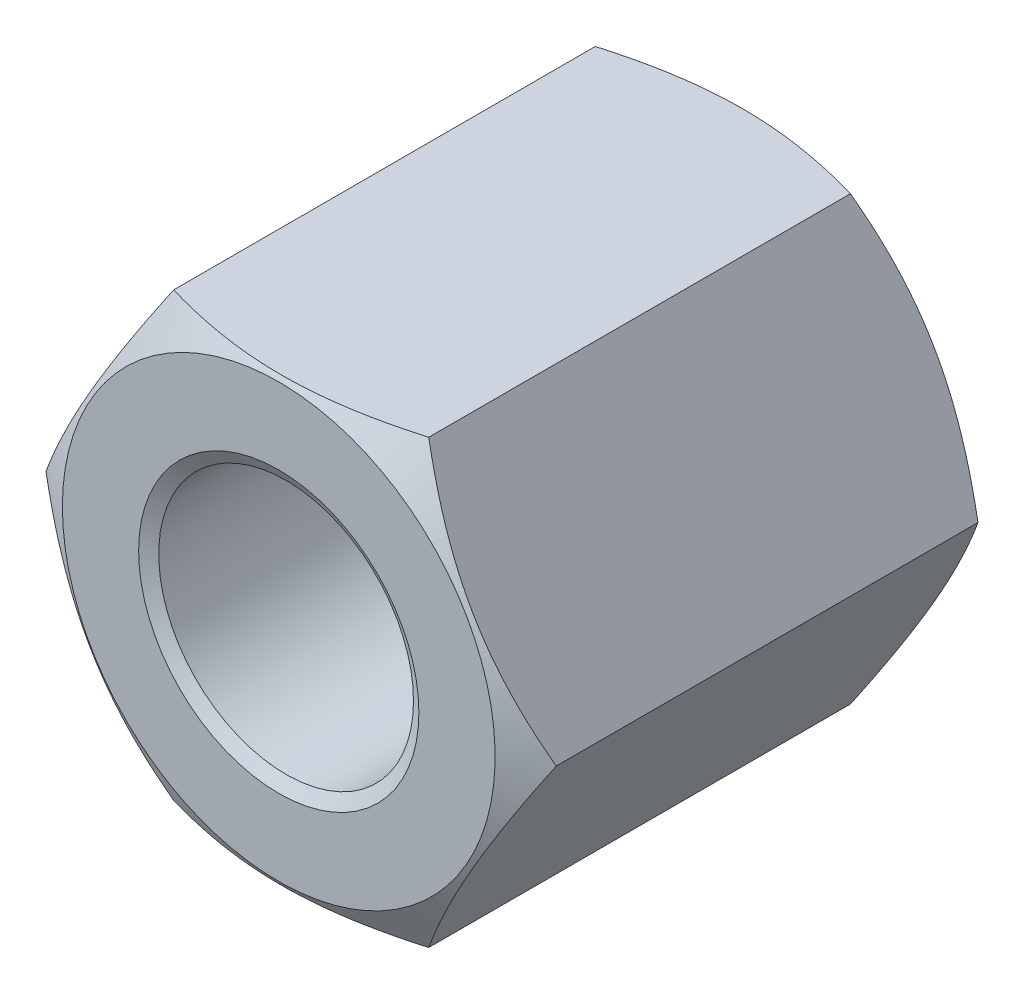
SolidWorks part; units mm, degrees
ref_plane "Front" through (0, 0, 0) normal (0, 0, 1) x (1, 0, 0)
ref_plane "Top" through (0, 0, 0) normal (0, 1, 0) x (1, 0, 0)
ref_plane "Right" through (0, 0, 0) normal (1, 0, 0) x (0, 0, -1)
other "Configuration Table"
sketch "Sketch1" plane through (0, 0, 0) normal (0, 0, 1) x (1, 0, 0)
  line L1 (10.3923, -18) -> (20.7846, 0)
  line L2 (20.7846, 0) -> (10.3923, 18)
  line L3 (10.3923, 18) -> (-10.3923, 18)
  line L4 (-10.3923, 18) -> (-20.7846, 0)
  line L5 (-20.7846, 0) -> (-10.3923, -18)
  line L6 (-10.3923, -18) -> (10.3923, -18)
  circle A0 centre (0, 0) radius 18 construction
  circle A1 centre (0, 0) radius 10.376
extrude "BaseNut" add sketch "Sketch1" against normal blind 38
cosmetic thread "ThreadCosmetic1" parameters "D2"=24
sketch "Sketch2" plane through (0, 0, 0) normal (0, 1, 0) x (1, 0, 0)
  line L0 (-20.7846, 38) -> (-17.625, 38)
  line L2 (-17.625, 38) -> (-20.7846, 36.1758)
  line L3 (-20.7846, 36.1758) -> (-20.7846, 38)
  line L4 (0, 3.3759) -> (0, -9.8171) construction
  line L6 (-9.7712, 19) -> (9.8853, 19) construction
  line L7 (-20.7846, 1.8242) -> (-20.7846, 0)
  line L8 (-17.625, 0) -> (-20.7846, 1.8242)
  line L9 (-20.7846, 0) -> (-17.625, 0)
revolve "Double-Chamfer" cut sketch "Sketch2" angle 360 about L4
chamfer "EndChamfer" distance 1.0376 angle 30 2 edges at (10.376, 0, 0) (10.376, 0, -38)
sketch "Sketch3" plane through (0, 0, 0) normal (0, 1, 0) x (1, 0, 0)
  line L0 (0, 28.565) -> (0, -12.1255) construction
  line L1 (8.752, 37.7744) -> (10.376, 37.7744)
  line L2 (10.376, 37.7744) -> (11.7824, 36.9624)
  line L3 (11.7824, 36.9624) -> (10.376, 36.1504)
  line L4 (10.376, 36.1504) -> (8.752, 36.1504)
  line L5 (8.752, 36.1504) -> (8.752, 37.7744)
  line L6 (10.376, 36.9624) -> (-10.376, 36.9624) construction
revolve "Cut-Revolve10" [suppressed] cut sketch "Sketch3" angle 360 about L0
pattern_linear "LPattern10" [suppressed] count 19 spacing 1.9488 along (0, 0, 1)
equation "\"dw@Sketch2\" = \"s@Sketch1\" - 0.75"
equation "\"D2@Sketch2\" = \"m@BaseNut\" / 2"
equation "\"D1@EndChamfer\" = \"D@Sketch1\" / 20"
equation "\"D1@Sketch3\" = (  \"D2@ThreadCosmetic1\" - \"D@Sketch1\" )  / 2"
equation "\"D2@Sketch3\" = \"D@Sketch1\""
equation "\"D3@LPattern10\" = \"D1@Sketch3\" * 1.2"
equation "\"D1@LPattern10\" = (  \"m@BaseNut\"  - \"D1@EndChamfer\")  / \"D3@LPattern10\" "
